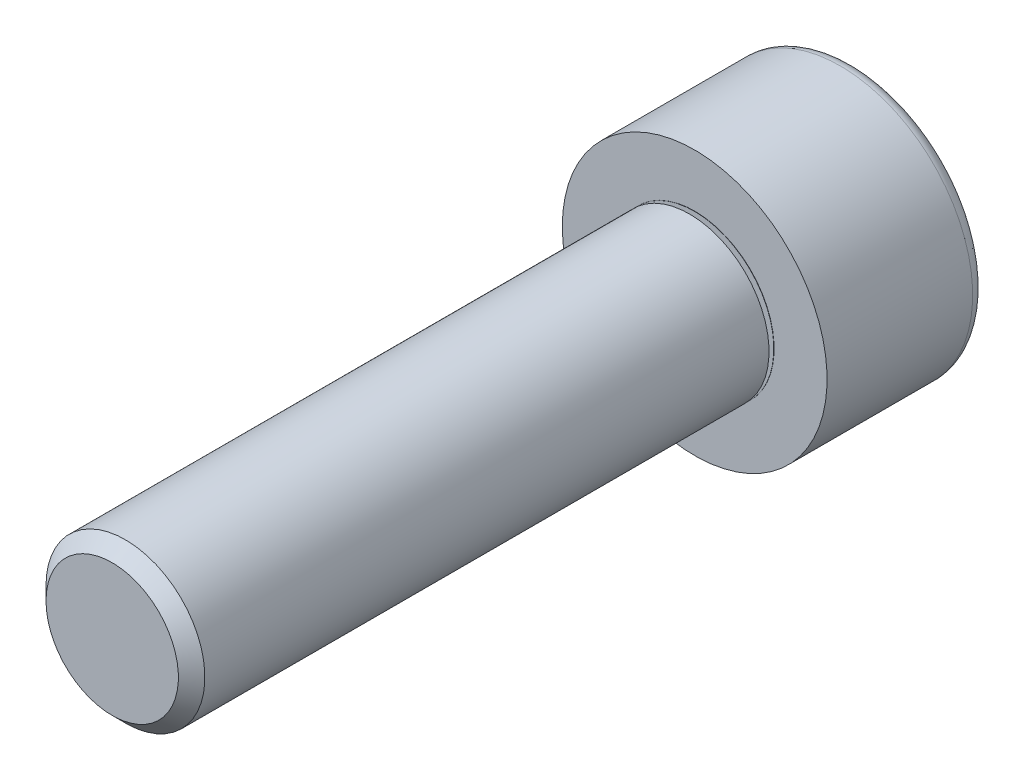
from build123d import *

# Parameters (mm, degrees)
CUT_EXTRUDE1_DEPTH = 2.5


with BuildPart() as part:
    # Logo3_bib1 → Revolve1 (revolve)
    with BuildSketch(Plane(origin=(0, 0, 0), x_dir=(-1, 0, 0), z_dir=(0, -1, 0))):
        with BuildLine():
            Line((0, -22), (0, 6))
            Line((0, 6), (4.5, 6))
            ThreePointArc((4.5, 6), (4.853553391, 5.853553391), (5, 5.5))
            Line((5, 5.5), (5, 0))
            Line((5, 0), (3, 0))
            Line((3, 0), (3, -0.01))
            Line((3, -0.01), (2.613425636, -0.01))
            ThreePointArc((2.613425636, -0.01), (2.593729481, -0.026527036), (2.606585234, -0.048793852))
            Line((2.606585234, -0.048793852), (3, -0.191985117))
            Line((3, -0.191985117), (3, -21.5))
            Line((3, -21.5), (2.5, -22))
            Line((2.5, -22), (0, -22))
        make_face()
    revolve(axis=Axis((0, 0, -10.585154653), (0, 0, 1)))

    # Logo3_bib2 → Cut-Extrude1 (cut)
    with BuildSketch(Plane(origin=(0, 0, -6), x_dir=(1, 0, 0), z_dir=(0, 0, -1))):
        Polygon((2.886751346, 0), (1.443375673, 2.5), (-1.443375673, 2.5), (-2.886751346, 0), (-1.443375673, -2.5), (1.443375673, -2.5), align=None)
    extrude(amount=-CUT_EXTRUDE1_DEPTH, mode=Mode.SUBTRACT)


solid = part.part
